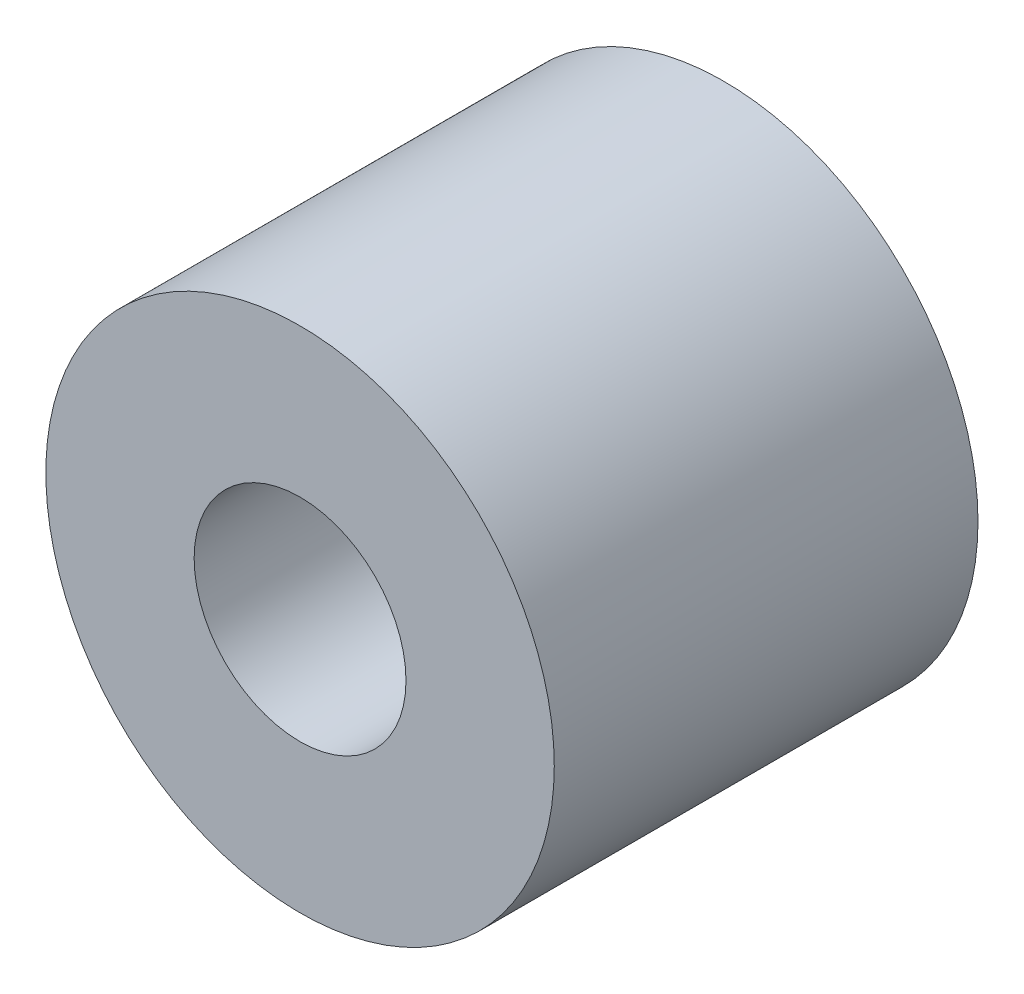
from build123d import *

# Parameters (mm, degrees)
SKETCH1_R           = 84
SKETCH1_R_2         = 35
BOSS_EXTRUDE1_DEPTH = 70


with BuildPart() as part:
    # Sketch1 → Boss-Extrude1 (new, symmetric)
    with BuildSketch(Plane.XY):
        Circle(SKETCH1_R)
        Circle(SKETCH1_R_2, mode=Mode.SUBTRACT)
    extrude(amount=BOSS_EXTRUDE1_DEPTH, both=True)


solid = part.part
